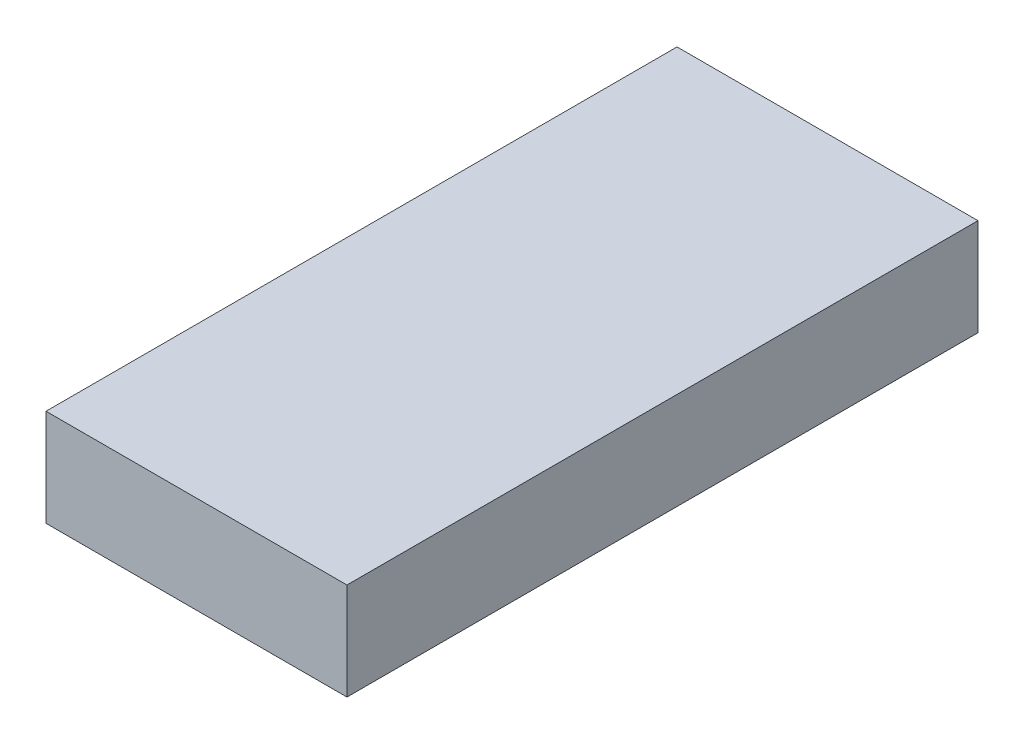
from build123d import *

# Parameters (mm, degrees)
SKETCH_1_W      = 310
SKETCH_1_H      = 650
EXTRUDE_1_DEPTH = 100


with BuildPart() as part:
    # 草图1 → 凸台-拉伸1 (new body)
    with BuildSketch(Plane(origin=(0, 0, 0), x_dir=(1, 0, 0), z_dir=(0, 1, 0))):
        Rectangle(SKETCH_1_W, SKETCH_1_H)
    extrude(amount=EXTRUDE_1_DEPTH)


solid = part.part
